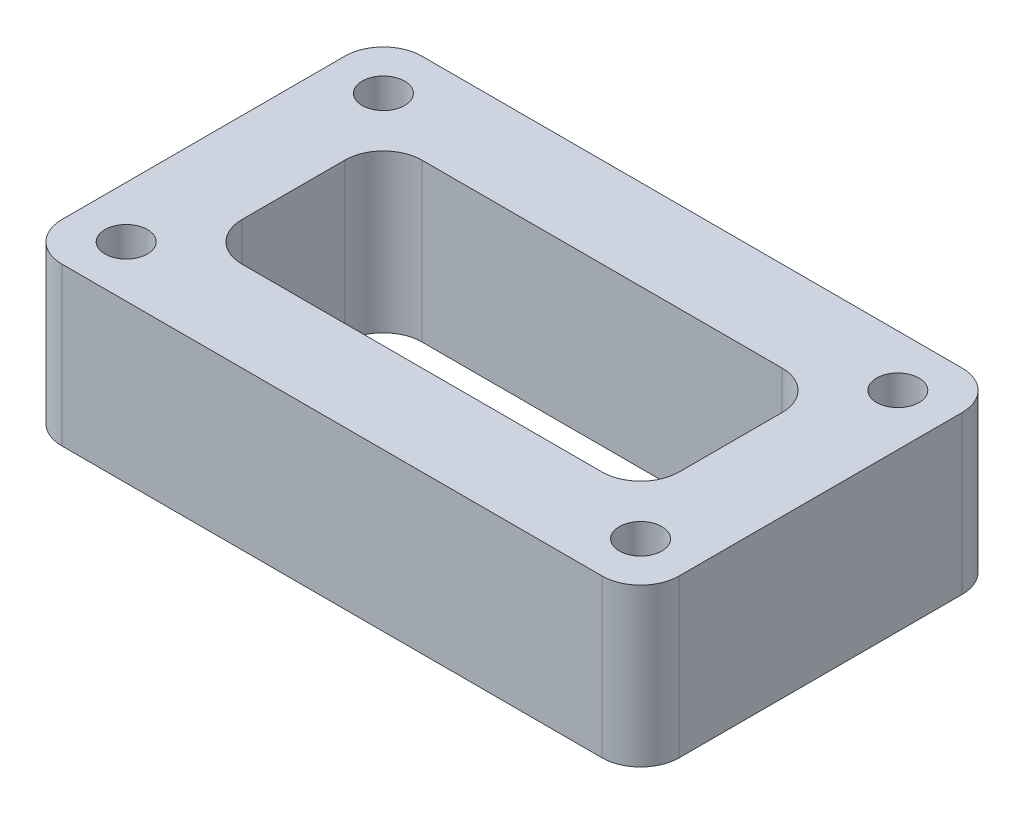
SolidWorks part; units mm, degrees
material "ABS"
ref_plane "前视基准面" through (0, 0, 0) normal (0, 0, 1) x (1, 0, 0)
ref_plane "上视基准面" through (0, 0, 0) normal (0, 1, 0) x (1, 0, 0)
ref_plane "右视基准面" through (0, 0, 0) normal (1, 0, 0) x (0, 0, -1)
other "Configuration Table"
sketch "草图1" plane through (0, 0, 0) normal (0, 1, 0) x (1, 0, 0)
  line L0 (-24, -11) -> (-24, 11)
  line L1 (-20, -10) -> (20, -10) construction
  line L2 (-20, -10) -> (-20, 10) construction
  line L3 (-20, 10) -> (20, 10) construction
  line L4 (20, -10) -> (20, 10) construction
  line L5 (-20, -10) -> (20, 10) construction
  line L6 (-20, 10) -> (20, -10) construction
  line L7 (-21, 14) -> (21, 14)
  line L8 (24, -11) -> (24, 11)
  line L9 (-21, -14) -> (21, -14)
  line L10 (-17, -4) -> (-17, 4)
  line L11 (-14, 7) -> (14, 7)
  line L12 (17, -4) -> (17, 4)
  line L13 (-14, -7) -> (14, -7)
  line L14 (24, -14) -> (24, 14) construction
  line L15 (-24, -14) -> (24, -14) construction
  line L16 (-24, 14) -> (24, 14) construction
  line L17 (-24, -14) -> (-24, 14) construction
  line L18 (-17, 7) -> (17, 7) construction
  line L19 (17, -7) -> (17, 7) construction
  line L20 (-17, -7) -> (-17, 7) construction
  line L21 (-17, -7) -> (17, -7) construction
  circle A0 centre (-20, 10) radius 1.65
  circle A1 centre (-20, -10) radius 1.65
  circle A2 centre (20, -10) radius 1.65
  circle A3 centre (20, 10) radius 1.65
  arc A4 (24, -11) -> (21, -14) centre (21, -11) cw
  arc A5 (21, 14) -> (24, 11) centre (21, 11) cw
  arc A6 (-24, 11) -> (-21, 14) centre (-21, 11) cw
  arc A7 (-24, -11) -> (-21, -14) centre (-21, -11) ccw
  arc A8 (14, 7) -> (17, 4) centre (14, 4) cw
  arc A9 (-17, -4) -> (-14, -7) centre (-14, -4) ccw
  arc A10 (-17, 4) -> (-14, 7) centre (-14, 4) cw
  arc A11 (17, -4) -> (14, -7) centre (14, -4) cw
  point P0 (0, 0)
  point P19 (0, 0)
  dimension "D5" = 3.3
  dimension "D6" = 3
  dimension "D1" = 20
  dimension "D2" = 40
  dimension "D3" = 4
  dimension "D4" = 3
extrude "凸台-拉伸1" add sketch "草图1" along normal blind 12.25
